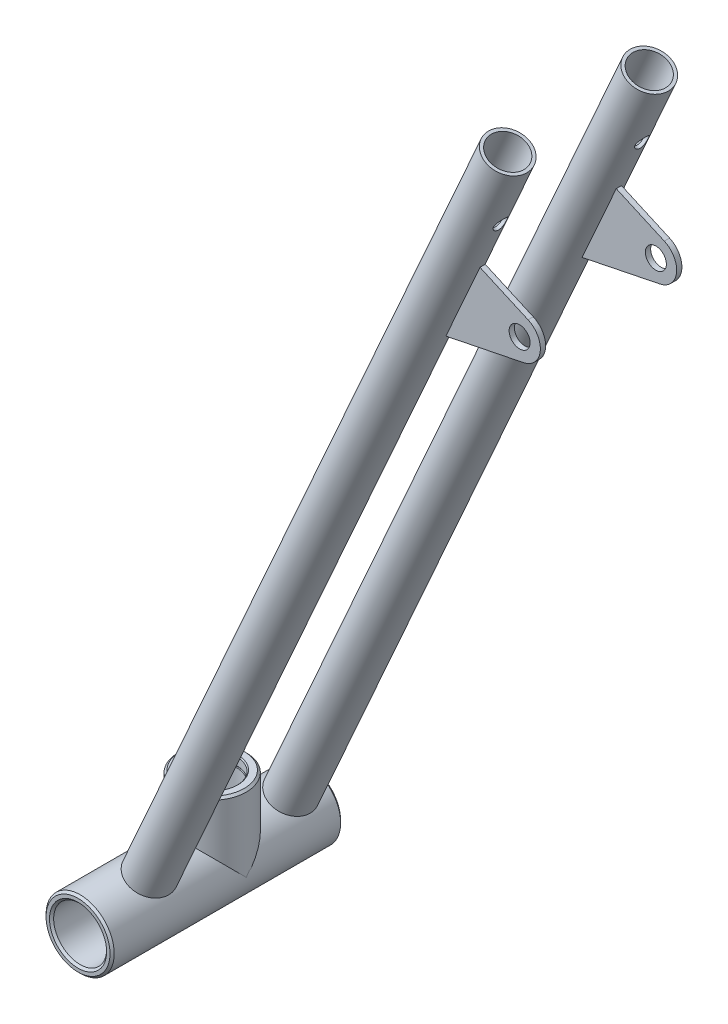
from build123d import *

# Parameters (mm, degrees)
SKETCH_1_R                     = 32.5
SKETCH_1_R_2                   = 25.25
EXTRUDE_1_DEPTH                = 220
EXTRUDE_2_REACH                = 247.929
EXTRUDE_2_END_RADIUS           = 32.5
SKETCH_3_R                     = 32.5
SKETCH_3_R_2                   = 23.5
SKETCH_4_R                     = 23.5
CUT_EXTRUDE_2_DEPTH            = 70
CHAMFER_1_SIZE                 = 2
CHAMFER_2_SIZE                 = 2
CHAMFER_3_SIZE                 = 1
SKETCH_5_R                     = 24.75
CUT_EXTRUDE_3_DEPTH            = 1.7
CHAMFER_4_SIZE                 = 2
SKETCH1_R                      = 20
SKETCH1_R_2                    = 17
GB_T6728_2002_42_3_X_3_1_DEPTH = 840
SKETCH_7_R                     = 6.5
CUT_EXTRUDE_6_DEPTH            = 25
SKETCH_8_R                     = 10
EXTRUDE_3_DEPTH                = 5


with BuildPart() as part:
    # 草图1 → 凸台-拉伸1 (new body)
    with BuildSketch(Plane.XY):
        Circle(SKETCH_1_R)
        Circle(SKETCH_1_R_2, mode=Mode.SUBTRACT)
    extrude(amount=EXTRUDE_1_DEPTH)

    # 草图4 → 切除-拉伸2 (cut)
    with BuildSketch(Plane(origin=(0, 72.5, 0), x_dir=(1, 0, 0), z_dir=(0, 1, 0))):
        with Locations(Location((0, -92, 0), (0, 0, 270))):
            Circle(SKETCH_4_R)
    extrude(amount=-CUT_EXTRUDE_2_DEPTH, mode=Mode.SUBTRACT)

    # 倒角2
    chamfer_2_edges = [part.edges().sort_by_distance(p)[0] for p in [
        (-32.5, 0, 0),
        (-32.5, 0, 220),
    ]]
    chamfer(chamfer_2_edges, length=CHAMFER_2_SIZE)

    # 倒角4
    chamfer_4_edges = [part.edges().sort_by_distance(p)[0] for p in [
        (-25.25, 0, 0),
        (-25.25, 0, 220),
    ]]
    chamfer(chamfer_4_edges, length=CHAMFER_4_SIZE)


with BuildPart() as body_2:
    # 凸台-拉伸2: up to this cylinder (the profile starts outside it)
    extrude_2_end = Plane(origin=(0, 0, 60.419239), z_dir=(0, 0, -1)) * Cylinder(EXTRUDE_2_END_RADIUS, 561.858, mode=Mode.PRIVATE)
    # 草图3 → 凸台-拉伸2 (new, up to the surface)
    with BuildSketch(Plane(origin=(0, 72.5, 0), x_dir=(1, 0, 0), z_dir=(0, 1, 0)), mode=Mode.PRIVATE) as extrude_2_sk1:
        with Locations(Location((0, -92, 0), (0, 0, 270))):
            Circle(SKETCH_3_R)
        with Locations(Location((0, -92, 0), (0, 0, 270))):
            Circle(SKETCH_3_R_2, mode=Mode.SUBTRACT)
    extrude_2_tool1 = extrude(extrude_2_sk1.sketch, amount=-EXTRUDE_2_REACH, mode=Mode.PRIVATE) - extrude_2_end
    add(extrude_2_tool1.solids().sort_by_distance((0, 72.5, 60.419239))[0])

    # 倒角1
    chamfer_1_edges = [body_2.edges().sort_by_distance(p)[0] for p in [
        (0, 72.5, 59.5),
    ]]
    chamfer(chamfer_1_edges, length=CHAMFER_1_SIZE)

    # 倒角3
    chamfer_3_edges = [body_2.edges().sort_by_distance(p)[0] for p in [
        (0, 72.5, 68.5),
    ]]
    chamfer(chamfer_3_edges, length=CHAMFER_3_SIZE)

    # 草图5 → 切除-拉伸3 (cut)
    with BuildSketch(Plane(origin=(0, 62.5, 0), x_dir=(1, 0, 0), z_dir=(0, 1, 0))):
        with Locations(Location((0, -92, 0), (0, 0, 270))):
            Circle(SKETCH_5_R)
    extrude(amount=CUT_EXTRUDE_3_DEPTH, mode=Mode.SUBTRACT)


with BuildPart() as body_3:
    # Sketch1 → 冷弯空心圆管gb∕t6728-2002 42.3 X 3(1) (new body)
    with BuildSketch(Plane(origin=(13.2189409, 29.690227373, 30), x_dir=(0.9135454576426006, -0.40673664307580093, 0), z_dir=(0.40673664307580093, 0.9135454576426006, 0))):
        Circle(SKETCH1_R)
        Circle(SKETCH1_R_2, mode=Mode.SUBTRACT)
    extrude(amount=GB_T6728_2002_42_3_X_3_1_DEPTH)

    # 草图7 → 切除-拉伸6 (cut, symmetric)
    with BuildSketch(Plane(origin=(0, 0, 0), x_dir=(0.40673664307580093, 0.9135454576426006, 0), z_dir=(0.9135454576426006, -0.40673664307580093, 0))):
        with Locations((812.5, 30)):
            Circle(SKETCH_7_R)
    extrude(amount=CUT_EXTRUDE_6_DEPTH, both=True, mode=Mode.SUBTRACT)


with BuildPart() as body_4:
    # 草图8 → 凸台-拉伸3 (new body)
    with BuildSketch(Plane(origin=(0, 0, 30), x_dir=(-1, 0, 0), z_dir=(0, 0, -1))):
        with BuildLine():
            Line((-328.407599498, 688.443678591), (-295.868668052, 615.36004198))
            Line((-295.868668052, 615.36004198), (-370.166624526, 630.527019722))
            ThreePointArc((-370.166624526, 630.527019722), (-385.894943686, 647.783914051), (-374.26120876, 668.028336422))
            Line((-374.26120876, 668.028336422), (-328.407599498, 688.443678591))
        make_face()
        with Locations((-366.204985914, 649.93376365)):
            Circle(SKETCH_8_R, mode=Mode.SUBTRACT)
    extrude(amount=-EXTRUDE_3_DEPTH)


with BuildPart() as body_5:
    # 镜向3: mirrored copy
    add(body_3.part.mirror(Plane(origin=(0, 0, 97.5), x_dir=(1, 0, 0), z_dir=(0, 0, -1))))


with BuildPart() as body_6:
    # Mirror 3 2: mirrored copy
    add(body_4.part.mirror(Plane(origin=(0, 0, 97.5), x_dir=(1, 0, 0), z_dir=(0, 0, -1))))


solid = Compound([part.part, body_2.part, body_3.part, body_4.part, body_5.part, body_6.part])
